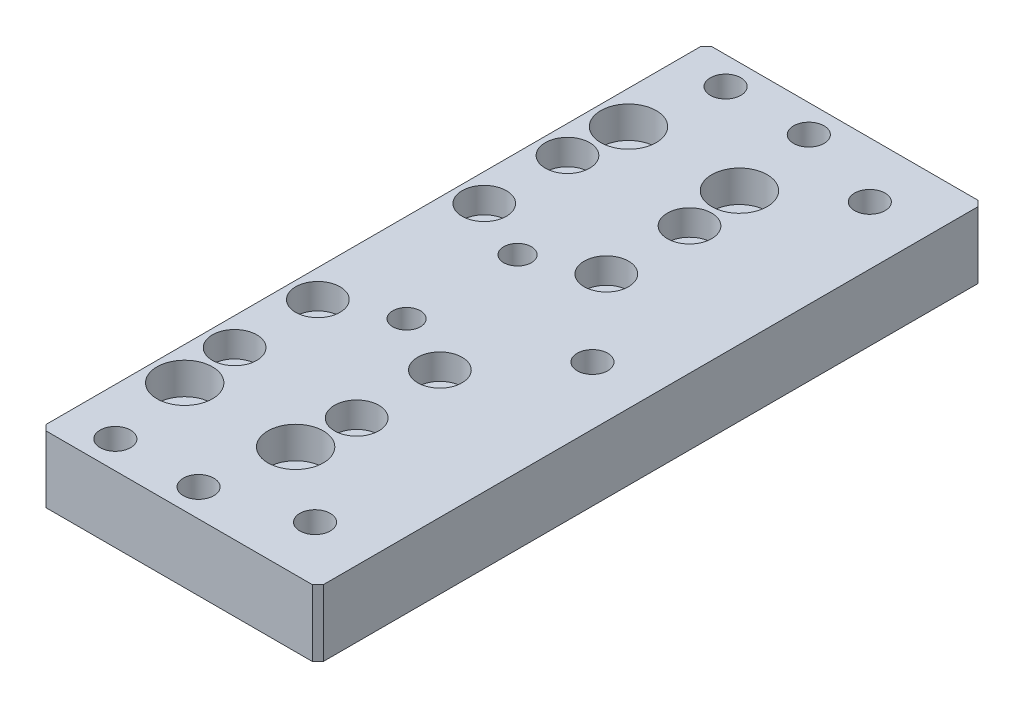
from build123d import *

# Parameters (mm, degrees)
SKETCH_1_W                   = 50
SKETCH_1_H                   = 120
EXTRUDE_1_DEPTH              = 6
HOLE_WIZARD_M4_1_D           = 4.5
HOLE_WIZARD_M4_1_CBORE_D     = 8
HOLE_WIZARD_M4_1_CBORE_DEPTH = 4.6
HOLE_WIZARD_M5_3_D           = 5.5
HOLE_WIZARD_M5_3_CBORE_D     = 9.5
HOLE_WIZARD_M5_3_CBORE_DEPTH = 5.7
HOLE_WIZARD_M6_1_D           = 5
HOLE_WIZARD_M6_1_DEPTH       = 15
HOLE_WIZARD_M6_1_TIP         = 1.502151548
HOLE_WIZARD_M5_1_D           = 5.5
HOLE_WIZARD_M5_1_CBORE_D     = 10
HOLE_WIZARD_M5_1_CBORE_DEPTH = 5.7
CHAMFER_1_SIZE               = 1
HOLE_WIZARD_M5_4_D           = 5.5
HOLE_WIZARD_M5_4_CBORE_D     = 10
HOLE_WIZARD_M5_4_CBORE_DEPTH = 5.7


with BuildPart() as part:
    # 草图1 → 凸台-拉伸1 (new, symmetric)
    with BuildSketch(Plane(origin=(0, 0, 0), x_dir=(1, 0, 0), z_dir=(0, 1, 0))):
        Rectangle(SKETCH_1_W, SKETCH_1_H)
    extrude(amount=EXTRUDE_1_DEPTH, both=True)

    # M4 六角圆柱头螺钉的柱形沉头孔1 (through all)
    with Locations(Plane(origin=(0, 6, 0), x_dir=(1, 0, 0), z_dir=(0, 1, 0))):
        with Locations((2, 15), (-20, 30), (2, 30), (-20, 15), (-20, -15), (2, -30), (-20, -30), (2, -15)):
            CounterBoreHole(HOLE_WIZARD_M4_1_D / 2, HOLE_WIZARD_M4_1_CBORE_D / 2, HOLE_WIZARD_M4_1_CBORE_DEPTH)

    # M5 六角圆柱头螺钉的柱形沉头孔3 (through all)
    with Locations(Plane(origin=(0, -6, 0), x_dir=(-1, 0, 0), z_dir=(0, -1, 0))):
        with Locations((16.499999999, -55), (1.500000001, -55), (1.500000001, 55), (16.499999999, 55)):
            CounterBoreHole(HOLE_WIZARD_M5_3_D / 2, HOLE_WIZARD_M5_3_CBORE_D / 2, HOLE_WIZARD_M5_3_CBORE_DEPTH)

    # M6 螺纹孔1
    with Locations(Plane(origin=(0, 6, 0), x_dir=(1, 0, 0), z_dir=(0, 1, 0))):
        with Locations((-9, 10), (-9, -10)):
            Hole(HOLE_WIZARD_M6_1_D / 2, depth=HOLE_WIZARD_M6_1_DEPTH)
            with Locations((0, 0, -(HOLE_WIZARD_M6_1_DEPTH + HOLE_WIZARD_M6_1_TIP / 2))):  # 118° drill point
                Cone(0, HOLE_WIZARD_M6_1_D / 2, HOLE_WIZARD_M6_1_TIP, mode=Mode.SUBTRACT)

    # M5 六角圆柱头螺钉的柱形沉头孔1 (through all)
    with Locations(Plane(origin=(0, 6, 0), x_dir=(1, 0, 0), z_dir=(0, 1, 0))):
        with Locations((1, 40), (1, -40), (-19, -40), (-19, 40)):
            CounterBoreHole(HOLE_WIZARD_M5_1_D / 2, HOLE_WIZARD_M5_1_CBORE_D / 2, HOLE_WIZARD_M5_1_CBORE_DEPTH)

    # 倒角1
    chamfer_1_edges = [part.edges().sort_by_distance(p)[0] for p in [
        (25, 0, 60),
        (-25, 0, 60),
        (-25, 0, -60),
        (25, 0, -60),
    ]]
    chamfer(chamfer_1_edges, length=CHAMFER_1_SIZE)

    # M5 六角圆柱头螺钉的柱形沉头孔4 (through all)
    with Locations(Plane(origin=(0, -6, 0), x_dir=(-1, 0, 0), z_dir=(0, -1, 0))):
        with Locations((-14.5, 50), (-14.5, 0), (-14.5, -50)):
            CounterBoreHole(HOLE_WIZARD_M5_4_D / 2, HOLE_WIZARD_M5_4_CBORE_D / 2, HOLE_WIZARD_M5_4_CBORE_DEPTH)


solid = part.part
